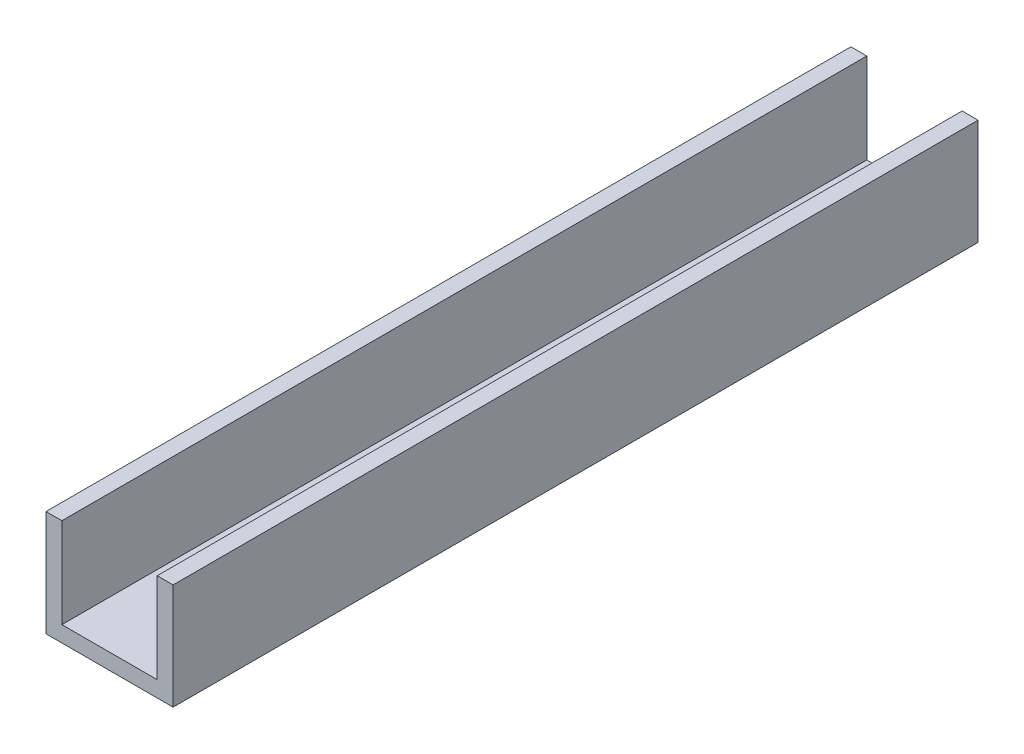
SolidWorks part; units mm, degrees
ref_plane "前视基准面" through (0, 0, 0) normal (0, 0, 1) x (1, 0, 0)
ref_plane "上视基准面" through (0, 0, 0) normal (0, 1, 0) x (1, 0, 0)
ref_plane "右视基准面" through (0, 0, 0) normal (1, 0, 0) x (0, 0, -1)
other "Configuration Table"
sketch "草图1" plane through (0, 0, 0) normal (0, 0, 1) x (1, 0, 0)
  line L0 (-6, -5) -> (6, -5)
  line L1 (6, -5) -> (6, 5)
  line L2 (6, 5) -> (4.5, 5)
  line L3 (4.5, 5) -> (4.5, -3.5)
  line L4 (4.5, -3.5) -> (-4.5, -3.5)
  line L5 (-4.5, -3.5) -> (-4.5, 5)
  line L6 (-4.5, 5) -> (-6, 5)
  line L7 (-6, 5) -> (-6, -5)
  point P0 (0, 0)
  dimension "D1" = 1.5
  dimension "D2" = 6
  dimension "D3" = 10.5
  dimension "D4" = 12
  dimension "D5" = 5
  dimension "D6" = 8.5
  dimension "D7" = 10
extrude "凸台-拉伸1" add sketch "草图1" against normal mid plane 90
sketch "草图2" plane through (0, 0, 0) normal (1, 0, 0) x (0, 0, -1)
  line L0 (-31, -6) -> (-31, 6)
  line L1 (-31, 6) -> (-46, 6)
  line L2 (-46, 6) -> (-46, -6)
  line L3 (-46, -6) -> (-31, -6)
  point P0 (0, 0)
  dimension "D1" = 15
  dimension "D2" = 46
  dimension "D3" = 6
  dimension "D4" = 12
extrude "切除-拉伸1" cut sketch "草图2" against normal mid plane 20
